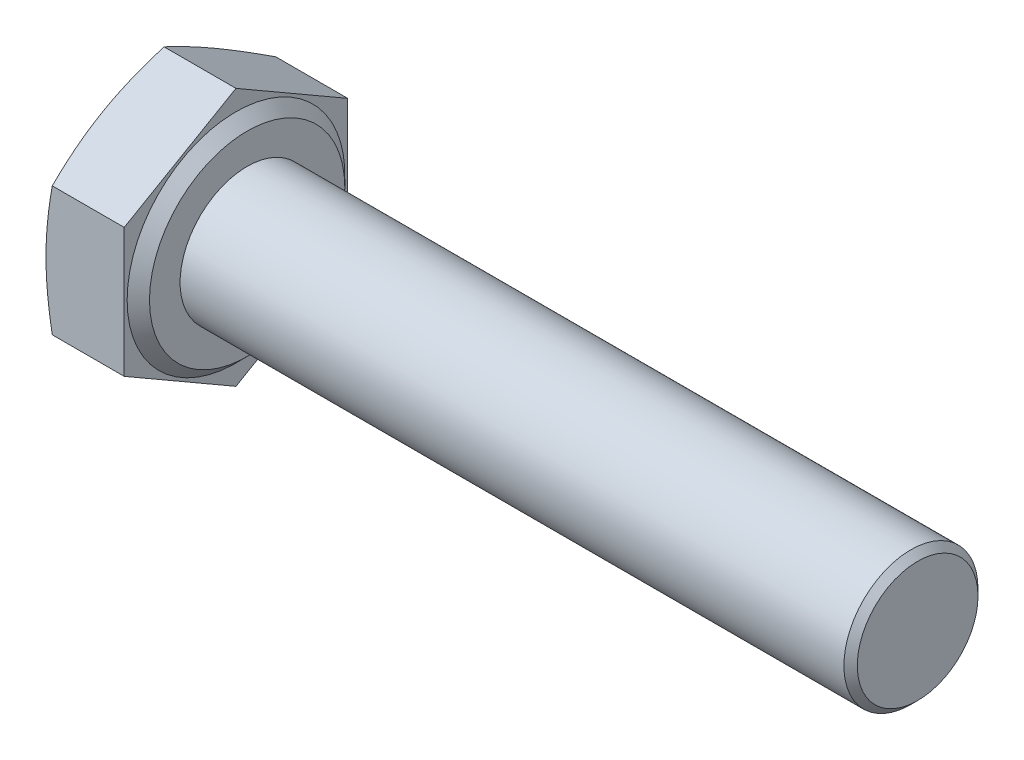
SolidWorks part; units mm, degrees
ref_plane "Front" through (0, 0, 0) normal (0, 0, 1) x (1, 0, 0)
ref_plane "Top" through (0, 0, 0) normal (0, 1, 0) x (1, 0, 0)
ref_plane "Right" through (0, 0, 0) normal (1, 0, 0) x (0, 0, -1)
other "Configuration Table"
sketch "Sketch2" plane through (0, 0, 0) normal (1, 0, 0) x (0, 0, -1)
  line L1 (0, -5.7735) -> (5, -2.8868)
  line L2 (5, -2.8868) -> (5, 2.8868)
  line L3 (5, 2.8868) -> (0, 5.7735)
  line L4 (0, 5.7735) -> (-5, 2.8868)
  line L5 (-5, 2.8868) -> (-5, -2.8868)
  line L6 (-5, -2.8868) -> (0, -5.7735)
  circle A0 centre (0, 0) radius 5 construction
extrude "BaseHead" add sketch "Sketch2" along normal blind 4
sketch "Sketch3" plane through (0, 0, 0) normal (0, 0, 1) x (1, 0, 0)
  line L0 (4, 5.7735) -> (4, 4.37)
  line L2 (4, 4.37) -> (3.5, 4.87)
  line L3 (3.5, 4.87) -> (3.5, 5.7735)
  line L5 (3.5, 5.7735) -> (4, 5.7735)
  line L6 (-0.9571, 0) -> (7.6478, 0) construction
  line L7 (4, 5.7735) -> (0, 5.7735) construction
  dimension "D1" = 45
  dimension "c" = 0.5
  dimension "dw" = 8.74
revolve "BearingFace" cut sketch "Sketch3" angle 360 about L6
sketch "Sketch4" plane through (0, 0, 0) normal (0, 0, 1) x (1, 0, 0)
  line L0 (-0.4935, 0) -> (3.5626, 0) construction
  line L2 (0, 5.7735) -> (0.2815, 5.7735)
  line L4 (0.2815, 5.7735) -> (0, 5)
  line L6 (0, 5) -> (0, 5.7735)
  line L7 (3.5, 5.7735) -> (0, 5.7735) construction
revolve "HeadChamfer" cut sketch "Sketch4" angle 360 about L0
sketch "Sketch5" plane through (4, 0, 0) normal (1, 0, 0) x (0, 0, -1)
  circle A0 centre (0, 0) radius 3
extrude "BaseBody" add sketch "Sketch5" along normal blind 30
cosmetic thread "ThreadCosmetic1" parameters "D2"=4.917
chamfer "Chamfer1" distance 0.3 angle 45 1 edges at (34, 0, -3)
fillet "HeadFillet" [suppressed] radius 0.25
sketch "Sketch6" plane through (0, 0, 0) normal (0, 0, 1) x (1, 0, 0)
  line L0 (4, 3.5415) -> (4.5415, 3.5415)
  line L1 (4.5415, 3.5415) -> (4.5415, 3)
  line L2 (4.5415, 3) -> (4.2708, 2.531)
  line L3 (4.2708, 2.531) -> (4, 3)
  line L4 (4, 3) -> (4, 3.5415)
  line L5 (4, -4.37) -> (4, 4.37) construction
  line L6 (33.7, 3) -> (4, 3) construction
revolve "Cut-Revolve10" [suppressed] cut sketch "Sketch6" angle 360
pattern_linear "LPattern10" [suppressed] count 46
equation "\"D2@Sketch4\" = \"s@Sketch2\""
equation "\"D1@Chamfer1\" = 0.05 * \"d@Sketch5\""
equation "\"D1@Sketch6\" =  ( \"d@Sketch5\" - \"D2@ThreadCosmetic1\" )  / 2"
equation "\"pitch@LPattern10\" = 1.2 * \"D1@Sketch6\""
equation "\"D1@LPattern10\" = (  \"l@BaseBody\"-\"D1@Chamfer1\" )  / \"pitch@LPattern10\""
